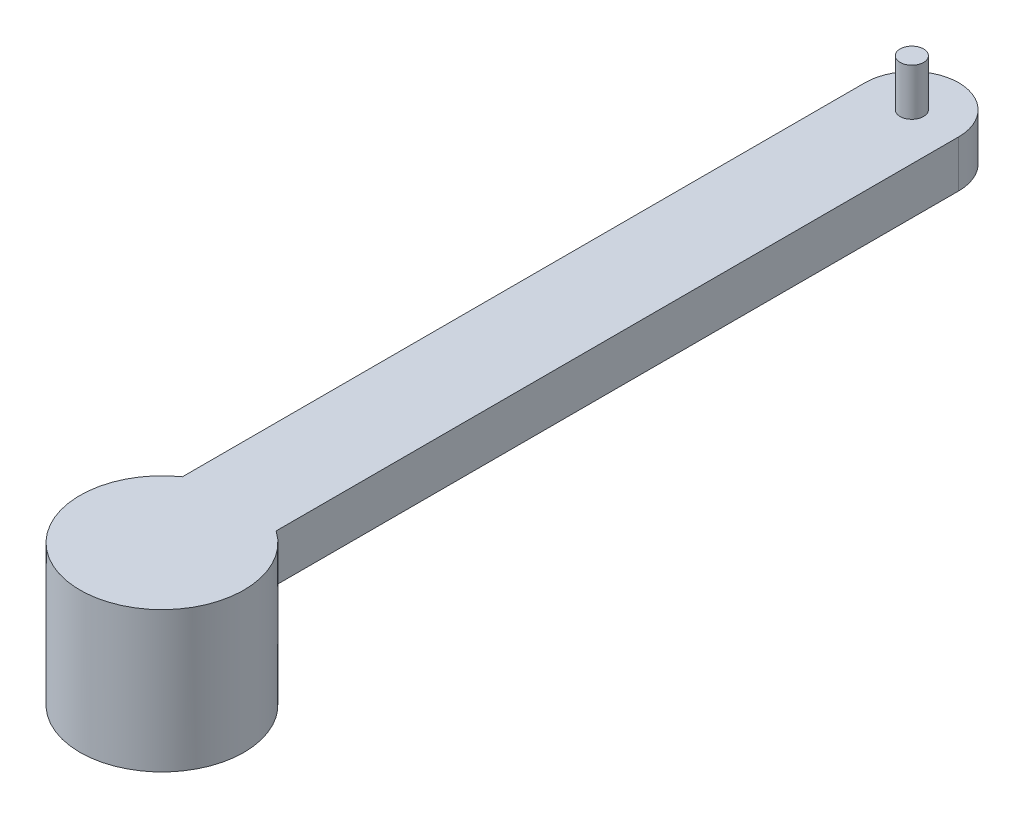
from build123d import *

# Parameters (mm, degrees)
SKETCH_1_R          = 17.5
EXTRUDE_1_DEPTH     = 30
SKETCH_2_R          = 5
CUT_EXTRUDE_1_DEPTH = 24
EXTRUDE_2_DEPTH     = 10
SKETCH_4_R          = 2.5
EXTRUDE_3_DEPTH     = 10


with BuildPart() as part:
    # 草图1 → 凸台-拉伸1 (new body)
    with BuildSketch(Plane(origin=(0, 0, 0), x_dir=(1, 0, 0), z_dir=(0, 1, 0))):
        with Locations(Location((0, 0, 0), (0, 0, 270))):
            Circle(SKETCH_1_R)
    extrude(amount=EXTRUDE_1_DEPTH)

    # 草图2 → 切除-拉伸1 (cut)
    with BuildSketch(Plane.XZ):
        with Locations(Location((0, 0, 0), (0, 0, 270))):
            Circle(SKETCH_2_R)
    extrude(amount=-CUT_EXTRUDE_1_DEPTH, mode=Mode.SUBTRACT)

    # 草图3 → 凸台-拉伸2 (add)
    with BuildSketch(Plane(origin=(0, 30, 0), x_dir=(1, 0, 0), z_dir=(0, 1, 0))):
        with BuildLine():
            Line((-10, 160), (-10, 0))
            Line((-10, 0), (10, 0))
            Line((10, 0), (10, 160))
            ThreePointArc((10, 160), (0, 170), (-10, 160))
        make_face()
    extrude(amount=-EXTRUDE_2_DEPTH)

    # 草图4 → 凸台-拉伸3 (add)
    with BuildSketch(Plane(origin=(0, 30, 0), x_dir=(1, 0, 0), z_dir=(0, 1, 0))):
        with Locations(Location((0, 160, 0), (0, 0, 270))):
            Circle(SKETCH_4_R)
    extrude(amount=EXTRUDE_3_DEPTH)


solid = part.part
